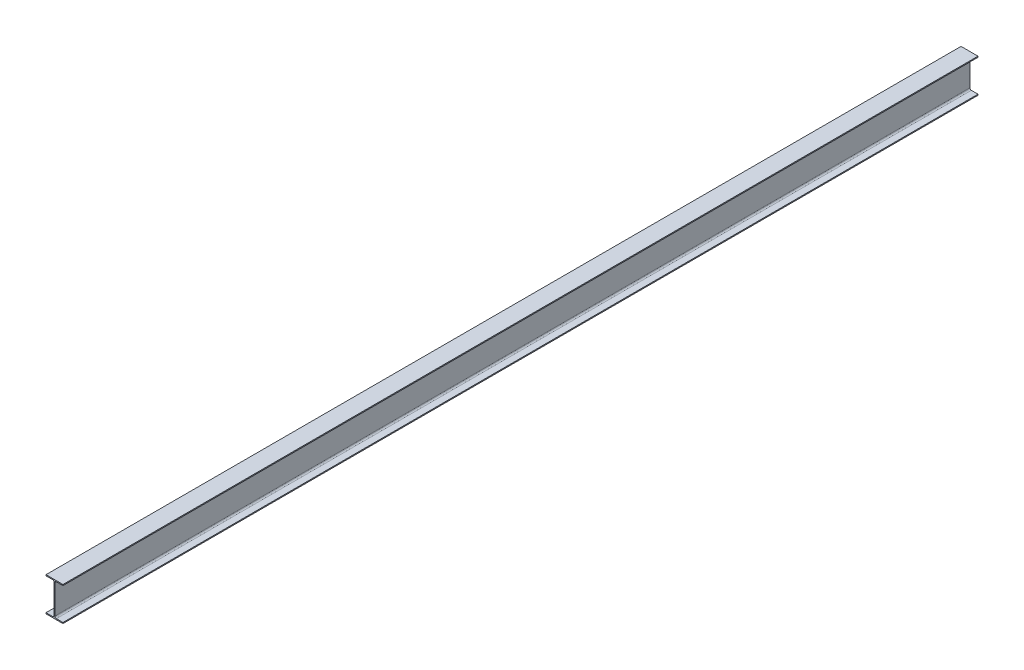
from build123d import *

# Parameters (mm, degrees)
BOSS_EXTRUDE1_DEPTH = 8090


with BuildPart() as part:
    # Sketch1 → Boss-Extrude1 (new body)
    with BuildSketch(Plane.XY):
        with BuildLine():
            Line((75, 0), (-75, 0))
            Line((-75, 0), (-75, 9))
            Line((-75, 9), (-16.25, 9))
            ThreePointArc((-16.25, 9), (-7.057611845, 12.807611845), (-3.25, 22))
            Line((-3.25, 22), (-3.25, 278))
            ThreePointArc((-3.25, 278), (-7.057611845, 287.192388155), (-16.25, 291))
            Line((-16.25, 291), (-75, 291))
            Line((-75, 291), (-75, 300))
            Line((-75, 300), (75, 300))
            Line((75, 300), (75, 291))
            Line((75, 291), (16.25, 291))
            ThreePointArc((16.25, 291), (7.057611845, 287.192388155), (3.25, 278))
            Line((3.25, 278), (3.25, 22))
            ThreePointArc((3.25, 22), (7.057611845, 12.807611845), (16.25, 9))
            Line((16.25, 9), (75, 9))
            Line((75, 9), (75, 0))
        make_face()
    extrude(amount=BOSS_EXTRUDE1_DEPTH)


solid = part.part
